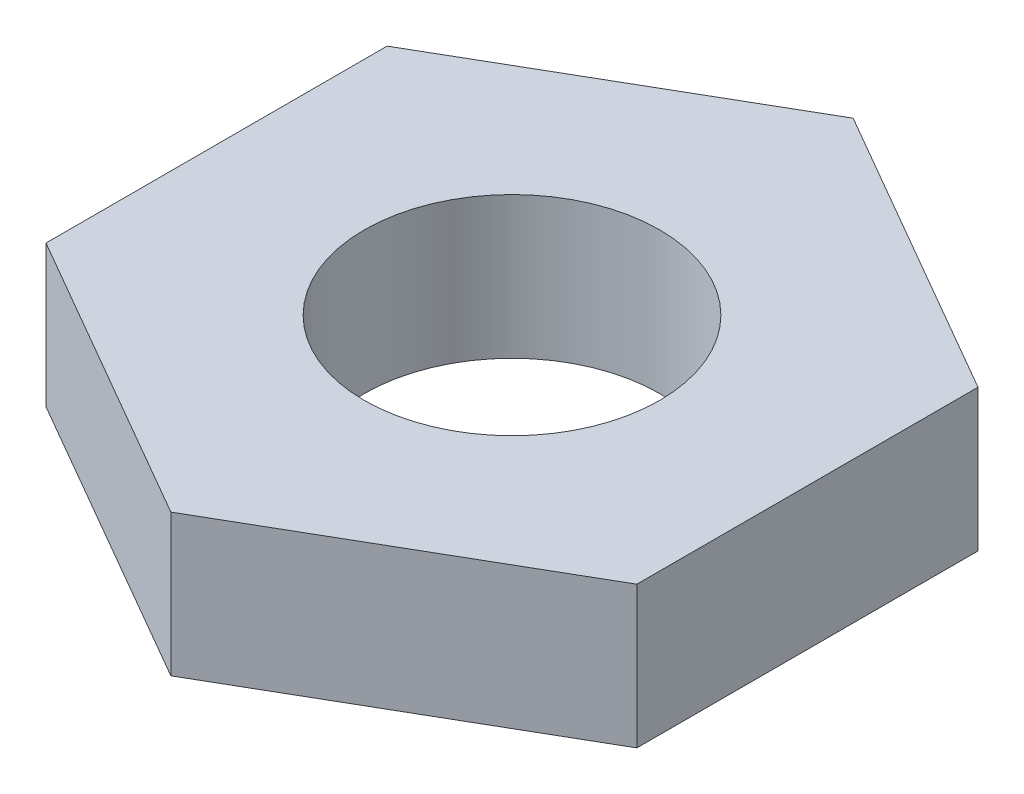
from build123d import *

# Parameters (mm, degrees)
EXTRUDE_1_DEPTH    = 2.4
HOLE_WIZARD_M6_1_D = 5


with BuildPart() as part:
    # 草图1 → 凸台-拉伸1 (new body)
    with BuildSketch(Plane(origin=(0, 0, 0), x_dir=(1, 0, 0), z_dir=(0, 1, 0))):
        Polygon((0, 5.773502692), (-5, 2.886751346), (-5, -2.886751346), (0, -5.773502692), (5, -2.886751346), (5, 2.886751346), align=None)
    extrude(amount=EXTRUDE_1_DEPTH)

    # M6 螺纹孔1 (through all)
    with Locations(Plane(origin=(0, 2.4, 0), x_dir=(1, 0, 0), z_dir=(0, 1, 0))):
        with Locations((0, 0)):
            Hole(HOLE_WIZARD_M6_1_D / 2)


solid = part.part
